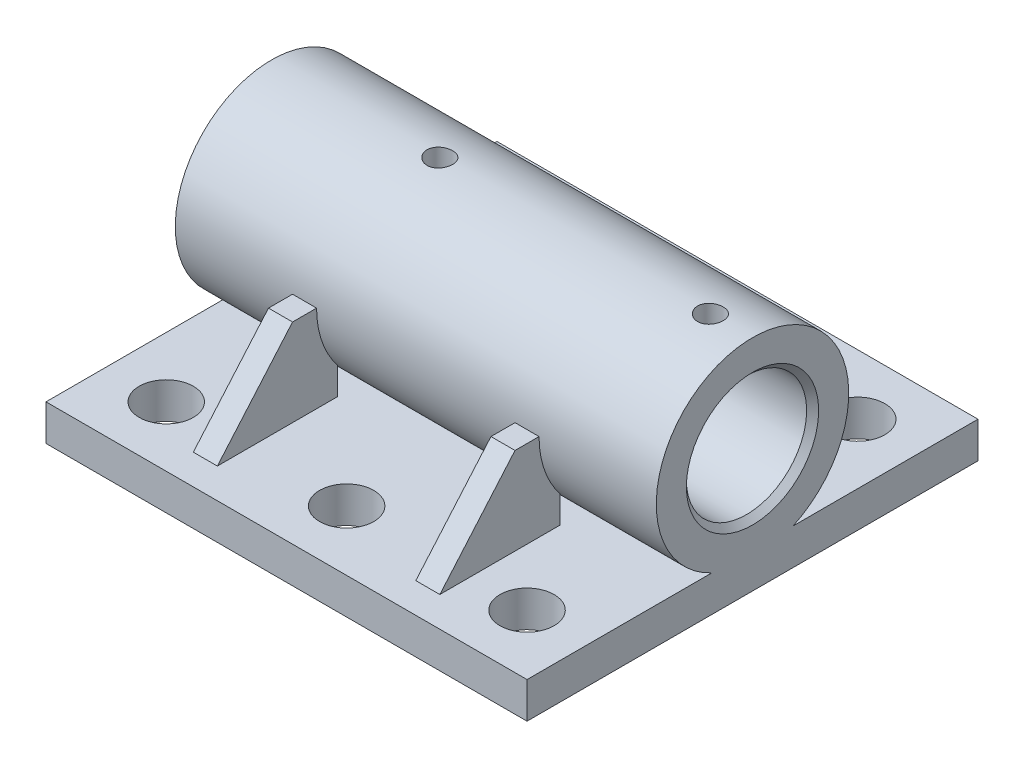
SolidWorks part; units mm, degrees
material "A3"
ref_plane "前视基准面" through (0, 0, 0) normal (0, 0, 1) x (1, 0, 0)
ref_plane "上视基准面" through (0, 0, 0) normal (0, 1, 0) x (1, 0, 0)
ref_plane "右视基准面" through (0, 0, 0) normal (1, 0, 0) x (0, 0, -1)
sketch "草图1" plane through (0, 0, 0) normal (0, 1, 0) x (1, 0, 0)
  line L0 (-60, -55) -> (0, -55) construction
  line L1 (-80, -75) -> (80, -75)
  line L2 (-80, -75) -> (-80, 75)
  line L3 (-80, 75) -> (80, 75)
  line L4 (80, -75) -> (80, 75)
  line L5 (-80, -75) -> (80, 75) construction
  line L6 (-80, 75) -> (80, -75) construction
  line L7 (-60, -55) -> (-60, 55) construction
  circle A0 centre (-60, -55) radius 9
  circle A1 centre (0, -55) radius 9
  circle A2 centre (60, -55) radius 9
  circle A3 centre (0, 55) radius 9
  circle A4 centre (60, 55) radius 9
  circle A5 centre (-60, 55) radius 9
  point P0 (0, 0)
  dimension "D3" = 18
  dimension "D5" = 55
  dimension "D1" = 150
  dimension "D2" = 160
  dimension "D4" = 20
  dimension "D8" = 60
  dimension "D9" = 110
  dimension "D6" = 3
  dimension "D7" = 2
extrude "凸台-拉伸1" add sketch "草图1" along normal blind 12
sketch "草图2" plane through (0, 0, 0) normal (0, 0, 1) x (1, 0, 0)
  line L0 (-77.9467, 41) -> (76.0867, 41) construction
  line L1 (-80, 0) -> (80, 0) construction
  line L2 (-80, 56) -> (-60, 56)
  line L3 (-60, 56) -> (-60, 64)
  line L4 (-60, 64) -> (40, 64)
  line L5 (40, 64) -> (40, 61)
  line L6 (40, 61) -> (80, 61)
  line L7 (80, 61) -> (80, 73)
  line L8 (80, 73) -> (-80, 73)
  line L9 (-80, 73) -> (-80, 56)
  line L10 (-80, 12) -> (-80, 0) construction
  line L11 (80, 12) -> (80, 0) construction
  dimension "D1" = 41
  dimension "D2" = 46
  dimension "D3" = 40
  dimension "D4" = 30
  dimension "D5" = 40
  dimension "D6" = 100
  dimension "D7" = 64
revolve "旋转1" add sketch "草图2" angle 360 about L0
sketch "草图4" plane through (0, 0, 0) normal (1, 0, 0) x (0, 0, -1)
  line L0 (-32, 41) -> (-40, 41)
  line L1 (-40, 41) -> (-65, 12)
  line L2 (-75, 12) -> (-13.5277, 12) construction
  line L3 (-65, 12) -> (-25, 12)
  line L4 (-25, 12) -> (-25, 21.025)
  line L5 (-75, 12) -> (-75, 0) construction
  arc A0 (13.5277, 12) -> (-13.5277, 12) centre (0, 41) ccw construction
  arc A1 (-32, 41) -> (-25, 21.025) centre (0, 41) ccw
  dimension "D1" = 8
  dimension "D2" = 10
  dimension "D3" = 40
extrude "凸台-拉伸2" add sketch "草图4" along normal blind 8 from offset 33 separate body
mirror "镜向1" about plane through (0, 0, 0) normal (0, 0, 1) of bodies 108
mirror "镜向2" about plane through (0, 0, 0) normal (1, 0, 0) of bodies 109 108
ref_plane "基准面1" through (0, 73, 0) normal (0, 1, 0) x (1, 0, 0)
hole_wizard "M10 螺纹孔1" positions "草图5" profile "草图6" tap size "M10" standard "GB"
sketch "草图5" plane through (0, 73, 0) normal (0, 1, 0) x (1, 0, 0)
  line L0 (-24, 0) -> (0, 0) construction
  line L4 (80, -32) -> (80, 32) construction
  point P0 (-24, 0)
  point P11 (66, 0)
  dimension "D1" = 90
  dimension "D2" = 14
sketch "草图6" plane through (-24, 73, 0) normal (1, 0, 0) x (0, 0, 1)
  line L0 (0, 0) -> (0, 30.0537)
  line L1 (0, 30.0537) -> (4.25, 27.5)
  line L2 (4.25, 27.5) -> (4.25, 0)
  line L5 (4.25, 0) -> (0, 0)
  line L10 (0, 30.0537) -> (-4.25, 27.5) construction
  line L11 (0, -6.35) -> (0, 107.95) construction
  dimension "螺纹孔钻头直径" = 8.5
  dimension "螺纹孔钻头深度" = 27.5
  dimension "导头角度" = 118
cosmetic thread "孔螺蚊线1" parameters "D1"=12.4568, "D2"=10
cosmetic thread "孔螺蚊线2" parameters "D1"=9.3961, "D2"=10
chamfer "倒角1" distance 1 angle 45 1 edges at (-80, 41, 15)
chamfer "倒角2" distance 2 angle 45 1 edges at (80, 41, 20)
